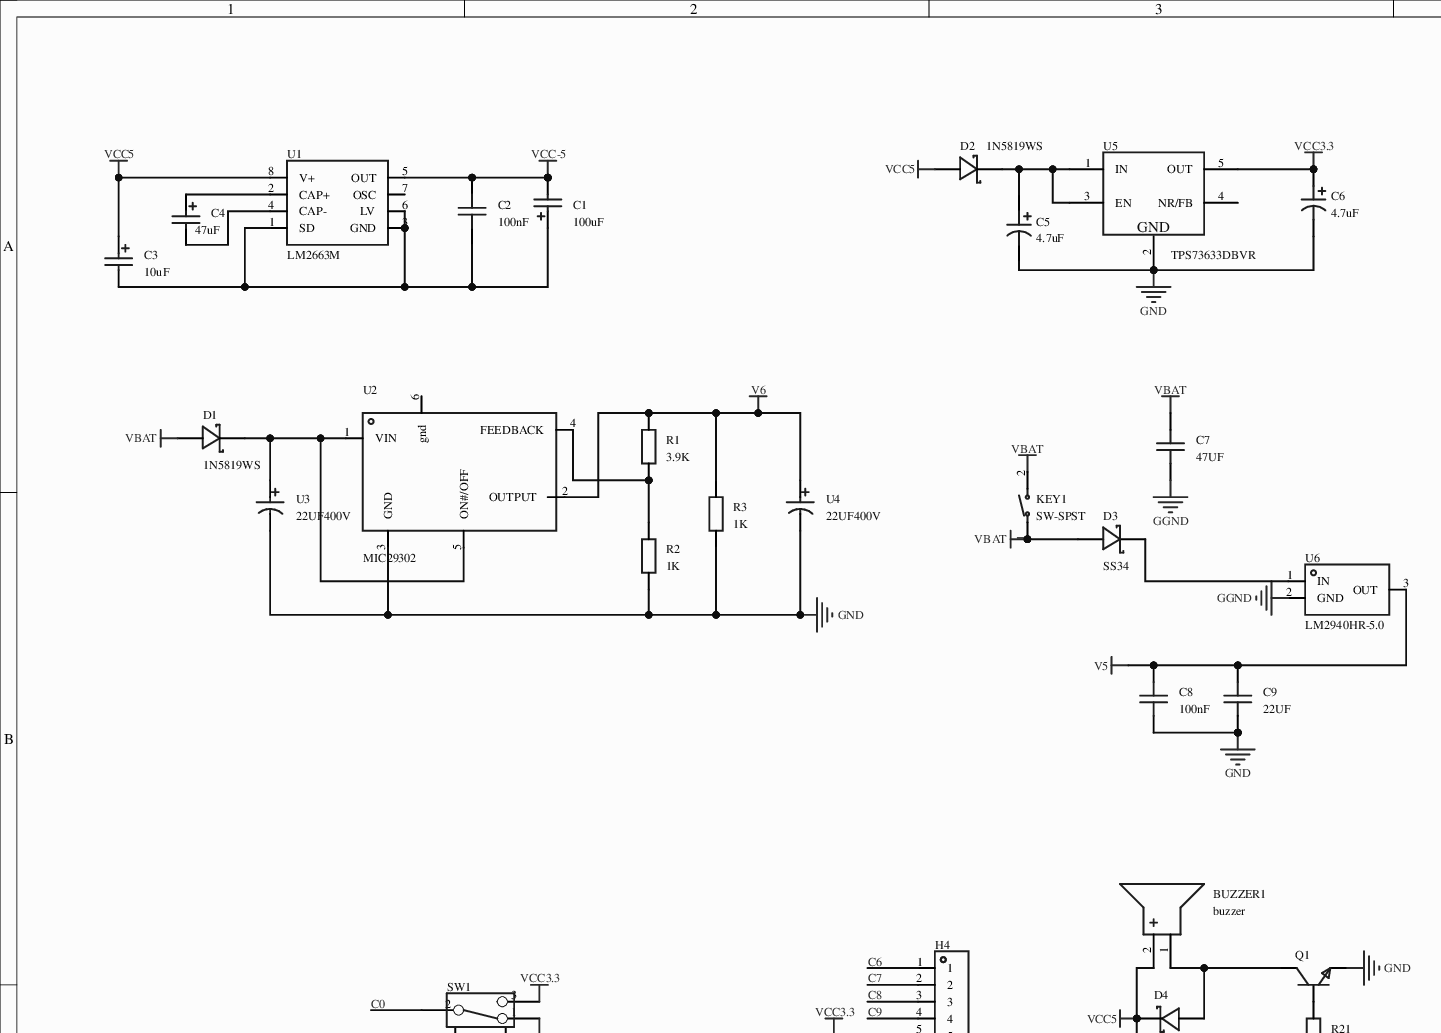
[diagram p0: MISC75407-3.schdoc, top left]
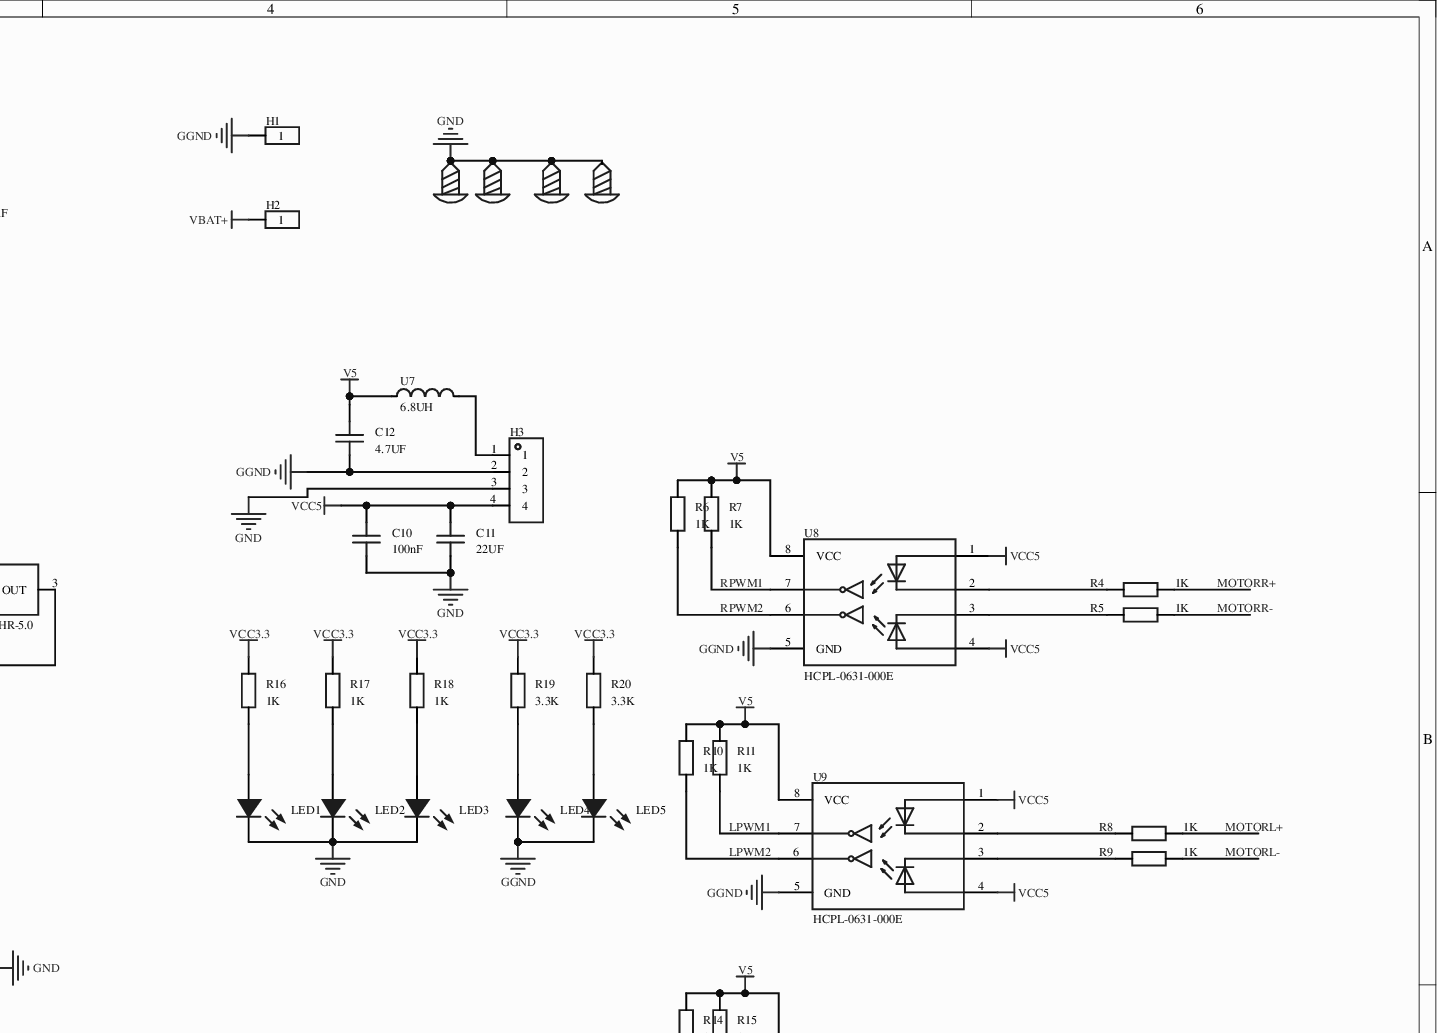
[diagram p1: MISC75407-3.schdoc, top right]
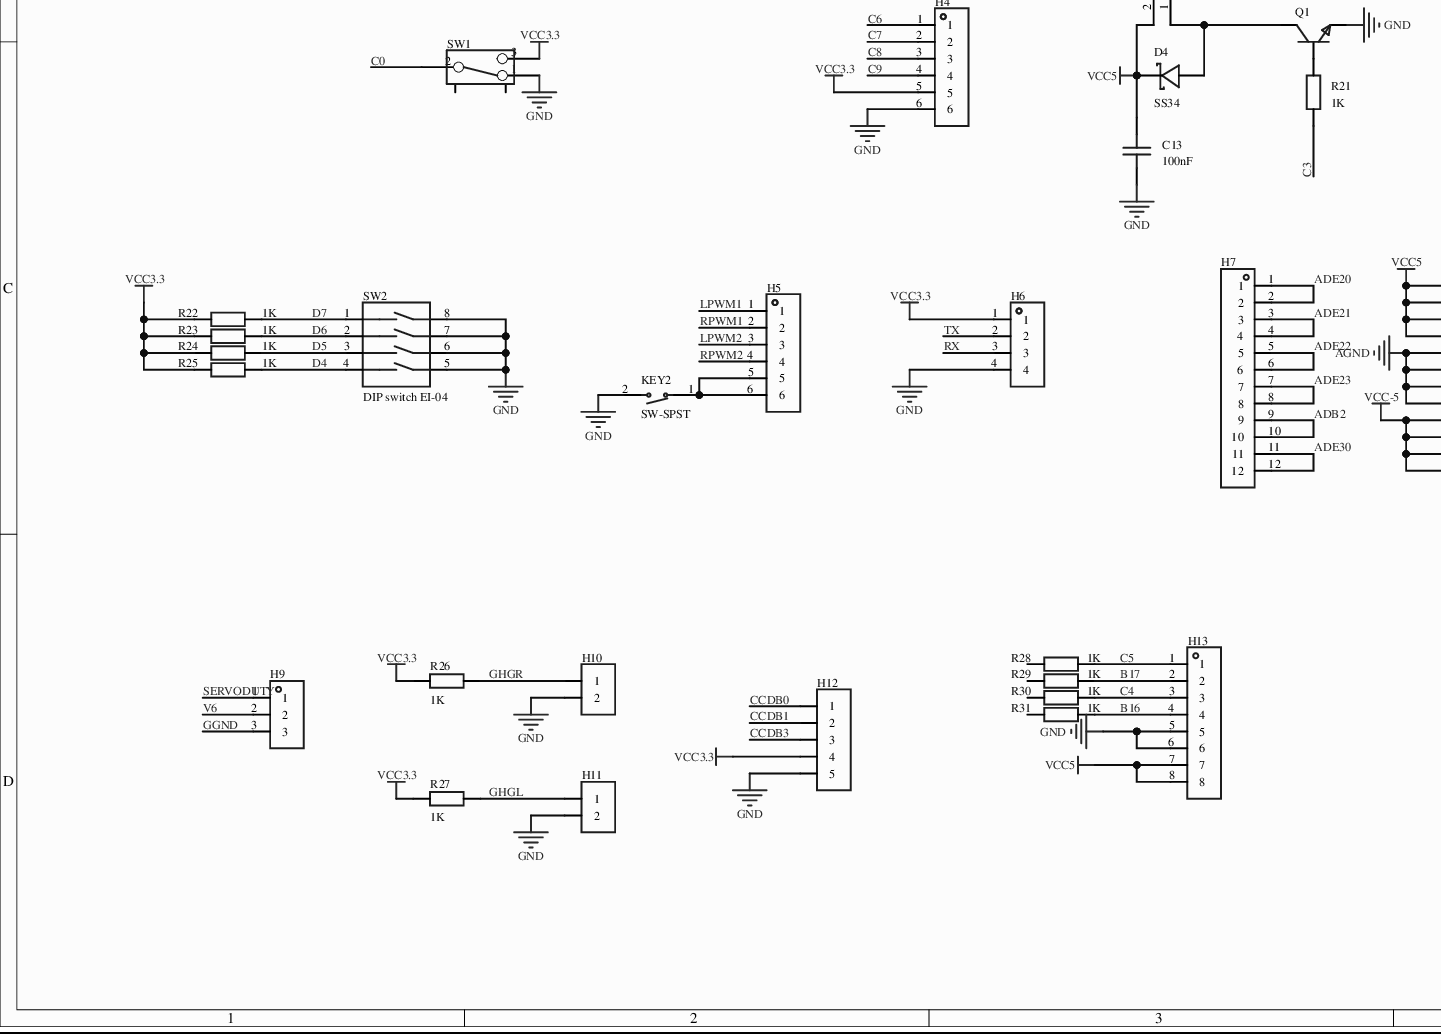
[diagram p2: MISC75407-3.schdoc, bottom left]
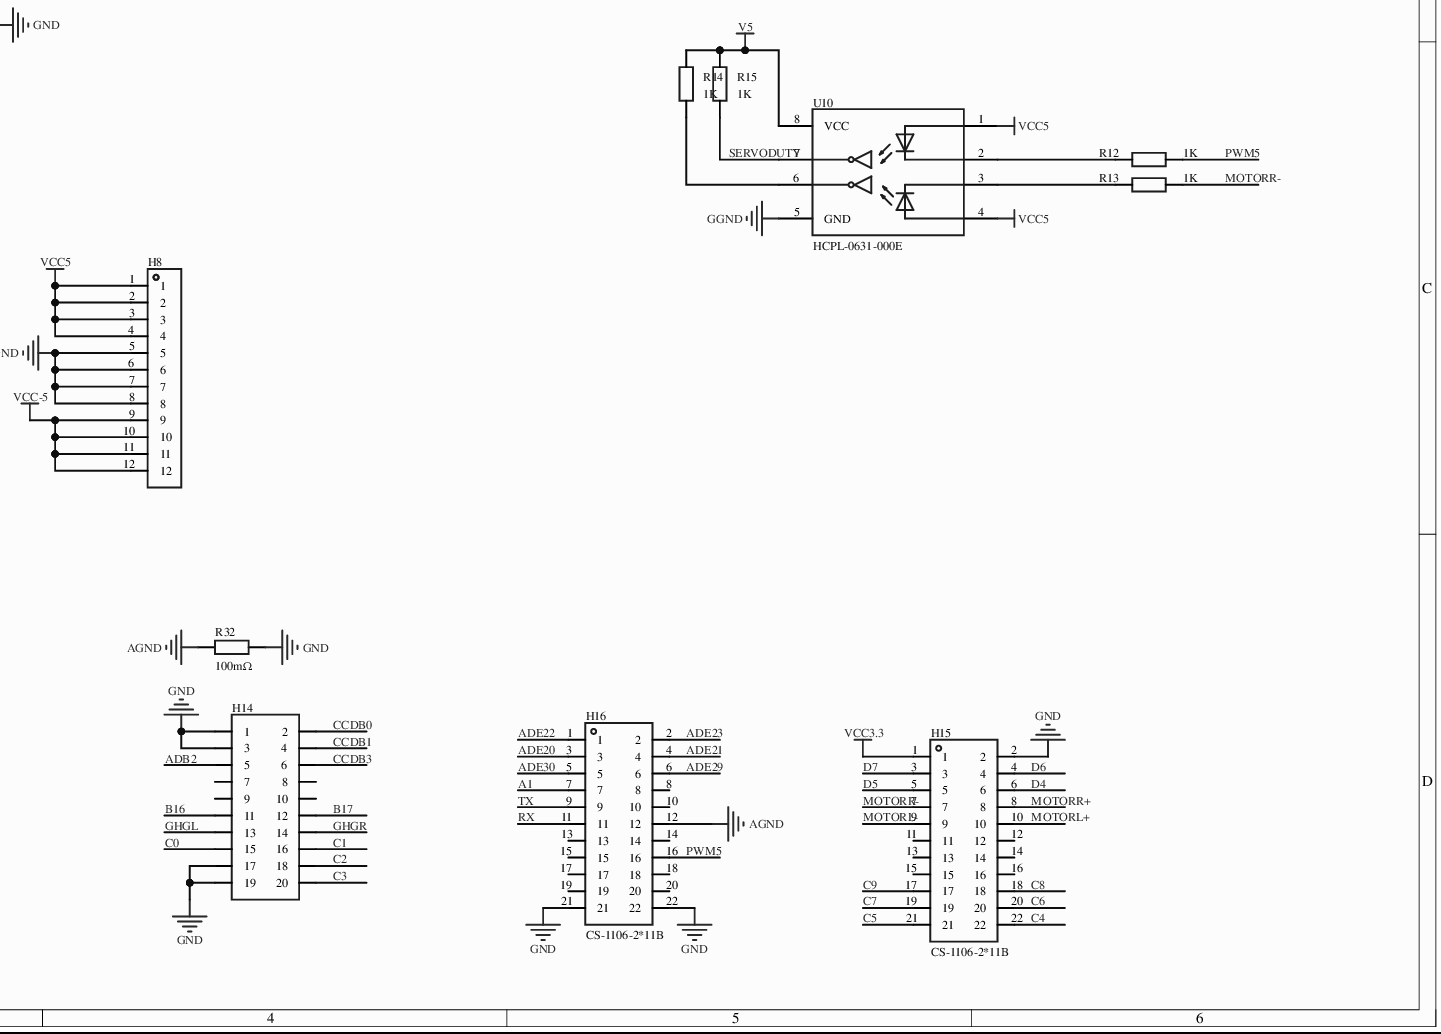
[diagram p3: MISC75407-3.schdoc, bottom right]
# Altium project MISC75407-2.PrjPcb
1 sheet, 90 parts. Net scope: global (net labels, ports and power ports of the same name join across sheets).
Board file: MISC75407.pcbdoc

## Sheet MISC75407-3.schdoc
size 420 x 297 mm; Version: V1.0; @Project Name: MISC75407; @Update Date: 2026-03-22; @Create Date: 2026-03-22; @Board Name: MISC75407; @Create Time: 21:34:52; @Page Count: 1; @Page No: 1; @Schematic Name: MISC75407; @Update Time: 21:34:52; Size: A4

### Parts
BUZZER1  buzzer  [BUZ-TH_BD12.0-P6.00-D0.9-RD]
C1  100uF  [C_Ele_SMD_3x5.4mm]
C2  100nF  [C0603]
C3  10uF  [C_Ele_SMD_3x5.4mm]
C4  47uF  [C_Ele_SMD_3x5.4mm]
C5  4.7uF  [CAP-TH_BD8.0-P3.50-D0.5-FD_4.7UF400V8X14FS]
C6  4.7uF  [CAP-TH_BD8.0-P3.50-D0.5-FD_4.7UF400V8X14FS]
C7  47UF  [C1206]
C8  100nF  [C0603]
C9  22UF  [C1206]
C10  100nF  [C0603]
C11  22UF  [C1206]
C12  4.7UF  [C0603]
C13  100nF  [C0603]
D1  1N5819WS  [SOD-323_L1.8-W1.3-LS2.5-RD]
D2  1N5819WS  [SOD-323_L1.8-W1.3-LS2.5-RD]
D3  SS34  [SMA_L4.3-W2.6-LS5.2-RD]
D4  SS34  [SMA_L4.3-W2.6-LS5.0-RD]
H1  (no value)  [HDR-TH_1P-V-M_XKB_X4611WV-01I-C28D40]
H2  (no value)  [HDR-TH_1P-V-M_XKB_X4611WV-01I-C28D40]
H3  (no value)  [HDR-TH_4P-P2.54-V-F]
H4  (no value)  [HDR-TH_6P-P2.54-V-F]
H5  (no value)  [HDR-TH_6P-P2.54-V-F]
H6  (no value)  [HDR-TH_4P-P2.54-V-F]
H7  (no value)  [HDR-TH_12P-P2.54-V-F]
H8  (no value)  [HDR-TH_12P-P2.54-V-F]
H9  (no value)  [HDR-TH_3P-P2.54-V-F]
H10  (no value)  [HDR-TH_2P-P2.54-V-F]
H11  (no value)  [HDR-TH_2P-P2.54-V-F]
H12  (no value)  [HDR-TH_5P-P2.54-V-F]
H13  (no value)  [HDR-TH_8P-P2.54-V-F-1]
H14  (no value)  [HDR-TH_20P-P2.54-V-R2-C10-S2.54]
H15  CS-1106-2*11B  [HDR-TH_22P-P2.54-V-M-R2-C11-S2.54-1]
H16  CS-1106-2*11B  [HDR-TH_22P-P2.54-V-M-R2-C11-S2.54-1]
KEY1  SW-SPST  [KEY-SMD_L6.0-W3.6-LS8.0]
KEY2  SW-SPST  [KEY-SMD_L6.0-W3.6-LS8.0]
LED1  (no value)  [LED-TH_5mm]
LED2  (no value)  [LED-TH_5mm]
LED3  (no value)  [LED-TH_5mm]
LED4  (no value)  [LED-TH_5mm]
LED5  (no value)  [LED-TH_5mm]
Q1  (no value)  [S8050_TO_92]
R1  3.9K  [R0603]
R2  1K  [R0603]
R3  1K  [R0603]
R4  1K  [R0603]
R5  1K  [R0603]
R6  1K  [R0603]
R7  1K  [R0603]
R8  1K  [R0603]
R9  1K  [R0603]
R10  1K  [R0603]
R11  1K  [R0603]
R12  1K  [R0603]
R13  1K  [R0603]
R14  1K  [R0603]
R15  1K  [R0603]
R16  1K  [R0603]
R17  1K  [R0603]
R18  1K  [R0603]
R19  3.3K  [R0603]
R20  3.3K  [R0603]
R21  1K  [R0603]
R22  1K  [R0603]
R23  1K  [R0603]
R24  1K  [R0603]
R25  1K  [R0603]
R26  1K  [R0603]
R27  1K  [R0603]
R28  1K  [R0603]
R29  1K  [R0603]
R30  1K  [R0603]
R31  1K  [R0603]
R32  100mΩ  [R1206]
SCREW1  (no value)  [M2螺丝]
SCREW2  (no value)  [M2螺丝]
SCREW3  (no value)  [M2螺丝]
SCREW4  (no value)  [M2螺丝]
SW1  (no value)  [拨动开关]
SW2  DIP switch EI-04  [SW-TH_DIPSWITCHEI-04]
U1  LM2663M  [SOIC-8_L4.9-W3.9-P1.27-LS6.0-BL]
U2  MIC29302  [TO-263-5_L10.1-W8.7-P1.70-LS15.2-BR]
U3  22UF400V  [CAP-TH_BD8.0-P3.50-D0.6-FD]
U4  22UF400V  [CAP-TH_BD8.0-P3.50-D0.6-FD]
U5  TPS73633DBVR  [SOT-23-5_L3.0-W1.7-P0.95-LS2.8-BR]
U6  LM2940HR-5.0  [TO-263-2_L10.1-W9.1-P5.08-LS15.2-BR]
U7  6.8UH  [IND-SMD_L10.9-W10.0_ACL1009]
U8  HCPL-0631-000E  [SO-8_L5.1-W3.9-P1.27-LS6.0-BL]
U9  HCPL-0631-000E  [SO-8_L5.1-W3.9-P1.27-LS6.0-BL]
U10  HCPL-0631-000E  [SO-8_L5.1-W3.9-P1.27-LS6.0-BL]

### Nets
AGND: H8.5 H8.6 H8.7 H8.8 H16.12 R32.1
GGND: C7.2 C12.1 H1.1 H3.2 H9.3 LED4.2(A) LED5.2(A) U6.2(GND) U8.5(GND) U9.5(GND) U10.5(GND)
GND: C5.2 C6.2 C8.1 C9.1 C10.1 C11.1 C13.1 H3.3 H4.6 H6.4 H10.2 H11.2 H12.5 H13.5 H13.6 H14.1 H14.3 H14.17 H14.19 H15.2 H16.21 H16.22 KEY2.2 LED1.2(A) LED2.2(A) LED3.2(A) Q1.1(E) R2.1 R3.1 R32.2 SCREW1.1 SCREW2.1 SCREW3.1 SCREW4.1 SW1.1 SW2.5 SW2.6 SW2.7 SW2.8 U2.3(GND) U3.2 U4.2 U5.2(GND)
V5: C8.2 C9.2 C12.2 R6.2 R7.2 R10.2 R11.2 R14.2 R15.2 U6.3(OUT) U7.1 U8.8(VCC) U9.8(VCC) U10.8(VCC)
V6: H9.2 R1.2 R3.2 U2.2(OUTPUT) U4.1
VBAT: C7.1 D1.2(A) D3.2(A) KEY1.1 KEY1.2
VBAT+: H2.1
VCC3.3: C6.1 H4.5 H6.1 H12.4 H15.1 R16.2 R17.2 R18.2 R19.2 R20.2 R22.1 R23.1 R24.1 R25.1 R26.1 R27.1 SW1.3 U5.5(OUT)
VCC5: BUZZER1.2(+) C3.1 C10.2 C11.2 C13.2 D2.2(A) D4.1(K) H3.4 H8.1 H8.2 H8.3 H8.4 H13.7 H13.8 U1.8(V+) U8.1(AN1) U8.4(AN2) U9.1(AN1) U9.4(AN2) U10.1(AN1) U10.4(AN2)
VCC-5: C1.2 C2.2 H8.9 H8.10 H8.11 H8.12 U1.5(OUT)
A1: H16.7
ADB2: H7.9 H7.10 H14.5
ADE20: H7.1 H7.2 H16.3
ADE21: H7.3 H7.4 H16.4
ADE22: H7.5 H7.6 H16.1
ADE23: H7.7 H7.8 H16.2
ADE29: H16.6
ADE30: H7.11 H7.12 H16.5
B16: H13.4 H14.11 R31.2
B17: H13.2 H14.12 R29.2
C0: H14.15 SW1.2
C1: H14.16
C2: H14.18
C3: H14.20 R21.1
C4: H13.3 H15.22 R30.2
C5: H13.1 H15.21 R28.2
C6: H4.1 H15.20
C7: H4.2 H15.19
C8: H4.3 H15.18
C9: H4.4 H15.17
CCDB0: H12.1 H14.2
CCDB1: H12.2 H14.4
CCDB3: H12.3 H14.6
D4: H15.6 R25.2 SW2.4
D5: H15.5 R24.2 SW2.3
D6: H15.4 R23.2 SW2.2
D7: H15.3 R22.2 SW2.1
GHGL: H11.1 H14.13 R27.2
GHGR: H10.1 H14.14 R26.2
LPWM1: H5.1 R11.1 U9.7(VO1)
LPWM2: H5.3 R10.1 U9.6(VO2)
MOTORL+: H15.10 R8.2
MOTORL-: H15.9 R9.2
MOTORR+: H15.8 R4.2
MOTORR-: H15.7 R5.2 R13.2
PWM5: H16.16 R12.2
RPWM1: H5.2 R7.1 U8.7(VO1)
RPWM2: H5.4 R6.1 U8.6(VO2)
RX: H6.3 H16.11
SERVODUTY: H9.1 R15.1 U10.7(VO1)
TX: H6.2 H16.9
NetBUZZER1_1: BUZZER1.1(-) D4.2(A) Q1.3(C)
NetC1_1: C1.1 C2.1 C3.2 U1.1(SD) U1.3(GND) U1.6(LV)
NetC4_1: C4.1 U1.2(CAP+)
NetC4_2: C4.2 U1.4(CAP-)
NetC5_1: C5.1 D2.1(K) U5.1(IN) U5.3(EN)
NetD1_1: D1.1(K) U2.1(VIN) U2.5(ON#/OFF) U3.1
NetD3_1: D3.1(K) U6.1(IN)
NetH3_1: H3.1 U7.2
NetH5_5: H5.5 H5.6 KEY2.1
NetLED1_1: LED1.1(C) R16.1
NetLED2_1: LED2.1(C) R17.1
NetLED3_1: LED3.1(C) R18.1
NetLED4_1: LED4.1(C) R19.1
NetLED5_1: LED5.1(C) R20.1
NetQ1_2: Q1.2(B) R21.2
NetR1_1: R1.1 R2.2 U2.4(FEEDBACK)
NetR4_1: R4.1 U8.2(CAT1)
NetR5_1: R5.1 U8.3(CAT2)
NetR8_1: R8.1 U9.2(CAT1)
NetR9_1: R9.1 U9.3(CAT2)
NetR12_1: R12.1 U10.2(CAT1)
NetR13_1: R13.1 U10.3(CAT2)
NetR14_1: R14.1 U10.6(VO2)

Not connected (* = marked no-connect by the designer): H14 7* 8* 9* 10*; H15 11* 12* 13* 14* 15* 16*; H16 8* 10* 13* 14* 15* 17* 18* 19* 20*; R28 1; R29 1; R30 1; R31 1; SW1 4 5; U1 7(OSC); U2 6(gnd); U5 4(NR/FB)

### Library data of the parts
BUZZER1 = buzzer: AddInBom: yes; ModelId: af17e4151ed84fc2a628230bf23763630819f05c4eef4c71ace90d822a990e87; ModelTransform: 472.44,472.176,0,270,0,0,0,0,-196.85; Symbol: BUZZER; Device: buzzer; LCSC Part Name: buzzer; SupplierPart: C9900014030; ManufacturerPart: buzzer; Supplier Footprint: buzzer; JLCPCB Part Class: Extended Part; Supplier: LCSC; ConvertToPcb: yes; FootprintName: BUZ-TH_BD12.0-P6.00-D0.9-RD; ModelName: BUZ-TH_BD12.0-P6.00-D0.9-RD
C1 C3 C4 = C_Ele_SMD_3x5.4mm: Symbol: CAP; AddInBom: yes; ModelId: 0132c3d3fdbf4fd987f710a97e7a5b5d0819f05c4eef4c71ace90d822a990e87; ModelName: CAP-SMD_BD3.0-L3.3-W3.3-H5.3; ModelTransform: 129.9,149.58,209.06,-90,0,0,0,0,0; Device: C_Ele_SMD_3x5.4mm; Supplier Footprint: SMD,3x5.4mm; ConvertToPcb: yes; FootprintName: C_Ele_SMD_3x5.4mm
  C1: Value: 100uF
  C3: Value: 10uF
  C4: Value: 47uF
C2 C8 C10 C12 C13 = CAP_0603: Symbol: Capacitance; ConvertToPcb: yes; ModelId: ac125912035d415993ca9572d50418b10819f05c4eef4c71ace90d822a990e87; ModelName: C0603_L1.6-W0.8-H0.8; ModelTransform: 62.992,31.496,0,0,0,0,0,0,0; Device: CAP_0603; AddInBom: yes; Supplier Footprint: 0603; FootprintName: C0603
  C2 C8 C10 C13: Value: 100nF
  C12: Value: 4.7UF
C5 C6 = 4.7uF400V8x14FS: Capacitance: 4.7uF; tolerance: ±20%; rated voltage: 400V; ripple current: 220mA@100KHz; equivalent series resistance (ESR): 11Ω;; Manufacturer: Econd(米朗电子); AddInBom: yes; Pin Spacing: 2.5mm; Lifetime: 5000hrs@105℃; Symbol: 4.7UF400V8X14FS; Device: 4.7uF400V8x14FS; LCSC Part Name: 4.7uF ±20% 400V; SupplierPart: C49304883; ManufacturerPart: 4.7uF400V8x14FS; Supplier Footprint: 插件,D8xL14mm; JLCPCB Part Class: Extended Part; Datasheet: https://item.szlcsc.com/datasheet/4.7uF400V8x14FS/51766711.html; Supplier: LCSC; ConvertToPcb: yes; FootprintName: CAP-TH_BD8.0-P3.50-D0.5-FD_4.7UF400V8X14FS; Value: 4.7uF; Tolerance: ±20%; Voltage Rating: 400V; Ripple Current: 220mA@100KHz; Equivalent Series Resistance(ESR): 11Ω; Diameter: 8mm; Height - Seated (Max): 14mm; Operating Temperature: -25℃~+105℃
C7 = 47UF: AddInBom: yes; ModelId: e4be705b945545a48e666415e3682bd80819f05c4eef4c71ace90d822a990e87; ModelName: C1206_L3.2-W1.6-H1.3; ModelTransform: 125.984,62.992,0,0,0,0,0,0,0; Symbol: 47UF; Device: 47UF; LCSC Part Name: 47UF; SupplierPart: C9900009812; ManufacturerPart: 47UF; Supplier Footprint: C1206; JLCPCB Part Class: Extended Part; Supplier: LCSC; ConvertToPcb: yes; FootprintName: C1206
C9 C11 = 22UF: Symbol: 22UF_C9900008064; AddInBom: yes; ModelId: e4be705b945545a48e666415e3682bd80819f05c4eef4c71ace90d822a990e87; ModelName: C1206_L3.2-W1.6-H1.3; ModelTransform: 125.984,62.992,0,0,0,0,0,0,0; Device: 22UF; LCSC Part Name: 22UF; SupplierPart: C9900008064; ManufacturerPart: 22UF; Supplier Footprint: 1206; JLCPCB Part Class: Extended Part; Supplier: LCSC; ConvertToPcb: yes; FootprintName: C1206
D1 D2 = 1N5819WS_C191023: Forward voltage (Vf): 600mV@1A; DC reverse voltage (Vr): 40V; rectified current: 1A;; Manufacturer: Hottech(合科泰); AddInBom: yes; ModelId: 7459fe65e23146c0a8d836e46a0add720819f05c4eef4c71ace90d822a990e87; ModelTransform: 104.3305,51.181,0,0,0,0,0,0,0; Non-Repetitive Peak Forward Surge Current: 25A; Symbol: 1N5819WS; Device: 1N5819WS_C191023; LCSC Part Name: 电压:40V 电流:1A; SupplierPart: C191023; ManufacturerPart: 1N5819WS; Supplier Footprint: SOD-323; JLCPCB Part Class: Basic Part; Datasheet: https://item.szlcsc.com/datasheet/1N5819WS/213850.html; Supplier: LCSC; ConvertToPcb: yes; FootprintName: SOD-323_L1.8-W1.3-LS2.5-RD; ModelName: SOD-323_L1.8-W1.3-LS2.5-RD; Voltage - Forward(Vf@If): 600mV@1A; Voltage - DC Reverse(Vr): 40V; Current - Rectified: 1A
D3 = SS34_C8678: Diode configuration: single; forward voltage (Vf): 550mV@3A; DC reverse voltage (Vr): 40V; rectified current: 3A;; Manufacturer: MDD(辰达半导体); AddInBom: yes; ModelId: e3551acb3c5a4975a5e9d36087fe1fa20819f05c4eef4c71ace90d822a990e87; ModelTransform: 185.039,102.362,0,0,0,0,0,0,0; Reverse Leakage Current (Ir): 500uA@40V; Operating Junction Temperature Range: -55℃~+125℃; Symbol: SS34_C8678; Device: SS34_C8678; LCSC Part Name: 电压:40V 电流:3A; SupplierPart: C8678; ManufacturerPart: SS34; Supplier Footprint: SMA(DO-214AC); JLCPCB Part Class: Basic Part; Datasheet: https://item.szlcsc.com/datasheet/SS34/9178.html; Supplier: LCSC; ConvertToPcb: yes; FootprintName: SMA_L4.3-W2.6-LS5.2-RD; ModelName: SMA_L4.3-W2.6-LS5.2-RD; Diode Configuration: Single; Voltage - Forward(Vf@If): 550mV@3A; Voltage - DC Reverse(Vr): 40V; Current - Rectified: 3A
D4 = SS34: Symbol: SS34_C9900023345; AddInBom: yes; ModelId: 8d2dd2e50a3a4b27821fa63d469a8f110819f05c4eef4c71ace90d822a990e87; ModelTransform: 196.85,102.362,0,0,0,0,0,0,0; Device: SS34; LCSC Part Name: SS34; SupplierPart: C9900023345; ManufacturerPart: SS34; Supplier Footprint: SMA,DO-214AC; JLCPCB Part Class: Extended Part; Supplier: LCSC; ConvertToPcb: yes; FootprintName: SMA_L4.3-W2.6-LS5.0-RD; ModelName: SMA_L4.3-W2.6-LS5.0-RD
H1 H2 = HDR-M_2.54_1x1P: Symbol: HDR_1x1; ConvertToPcb: yes; ModelId: 95857080d3cc4057a19a22ccce05e1710819f05c4eef4c71ace90d822a990e87; ModelTransform: 78.74,79.1337,0,0,0,0,0,0,-110.236; Device: HDR-M_2.54_1x1P; AddInBom: yes; SupplierPart: C81276; Supplier Footprint: 插件; FootprintName: HDR-TH_1P-V-M_XKB_X4611WV-01I-C28D40; JLCPCB Part Class: Extended Part; ModelName: HDR-TH_1P-V-M_XKB_X4611WV-01I-C28D40
H3 H6 = HDR-F_2.54_1x4P: Symbol: 2.54-1*4P female; ConvertToPcb: yes; ModelId: d187812051054f85879fcaa51a310d8e0819f05c4eef4c71ace90d822a990e87; ModelTransform: 419.6842,98.464,0,0,0,0,0,0,-118.11; Device: HDR-F_2.54_1x4P; AddInBom: yes; SupplierPart: C2718488; Supplier Footprint: 插件; FootprintName: HDR-TH_4P-P2.54-V-F; ModelName: HDR-TH_4P-P2.54-V-F
H4 H5 = HDR-F_2.54_1x6P: Symbol: Header-Female-2.54_1x6; ConvertToPcb: yes; ModelId: 0f5bcf94dcda47d085f24cdca1696fe90819f05c4eef4c71ace90d822a990e87; ModelTransform: 619.684,94.488,0,0,0,0,0,0,-125.984; Device: HDR-F_2.54_1x6P; AddInBom: yes; SupplierPart: C40877; Supplier Footprint: 插件; FootprintName: HDR-TH_6P-P2.54-V-F; ModelName: HDR-TH_6P-P2.54-V-F
H7 H8 = HDR-F_2.54_1x12P: ConvertToPcb: yes; ModelId: a8b4b2347edc4eeab5667ae97bf18e170819f05c4eef4c71ace90d822a990e87; ModelName: HDR-TH_12P-P2.54-F-LI-1X12P; ModelTransform: 1215.74568,98.425,0,0,0,0,0,0,-129.921; Symbol: HDR-F_2.54_1x12P; Device: HDR-F_2.54_1x12P; AddInBom: yes; SupplierPart: C2905419; Supplier Footprint: 插件; FootprintName: HDR-TH_12P-P2.54-V-F
H9 = HDR-F_2.54_1x3P: Symbol: PM254V-11-03-H85; ConvertToPcb: yes; ModelId: f3b3cc5aae9641bf9e56fc160cef875b0819f05c4eef4c71ace90d822a990e87; ModelName: HDR2.54-F-LI-1X3P; ModelTransform: 299.9994,100,0,0,0,0,0,0,-118.11; Device: HDR-F_2.54_1x3P; AddInBom: yes; SupplierPart: C541850; Supplier Footprint: 插件; FootprintName: HDR-TH_3P-P2.54-V-F
H10 H11 = HDR-F_2.54_1x2P: Symbol: Header-Female-2.54_1x2; ConvertToPcb: yes; ModelId: a9450ef445564560a104363b9aacde4e0819f05c4eef4c71ace90d822a990e87; ModelName: HDR-TH_2P-P2.54-F-LI-1X2P; ModelTransform: 215.7476,98.425,0,0,0,0,0,0,-129.921; Device: HDR-F_2.54_1x2P; AddInBom: yes; SupplierPart: C49661; Supplier Footprint: 插件; FootprintName: HDR-TH_2P-P2.54-V-F
H12 = HDR-F_2.54_1x5P: Symbol: Header-Female-2.54_1x5; ConvertToPcb: yes; ModelId: f49cb6116a3d45e5a64915bf3e00773f0819f05c4eef4c71ace90d822a990e87; ModelTransform: 519.684,98.464,0,0,0,0,0,0,-124.016; Device: HDR-F_2.54_1x5P; AddInBom: yes; SupplierPart: C50950; Supplier Footprint: 插件; FootprintName: HDR-TH_5P-P2.54-V-F; ModelName: HDR-TH_5P-P2.54-V-F
H13 = HDR-F_2.54_1x8P: Symbol: Header-Female-2.54_1x8; AddInBom: yes; ModelId: 0f7e4d9227ef4fa08d5469c22cc70cdb0819f05c4eef4c71ace90d822a990e87; ModelName: HDR-F-2.54_1x8; ModelTransform: 799.99844,100,0,0,0,0,0,0,-118.11; Device: HDR-F_2.54_1x8P; ConvertToPcb: yes; FootprintName: HDR-TH_8P-P2.54-V-F-1; SupplierPart: C27438; Supplier Footprint: 插件
H14 = HDR-F_2.54_2x10: Symbol: HDR-F-2.54_2x10; ConvertToPcb: yes; ModelId: e61a236d230547b1b0067fd6f2acc5ad0819f05c4eef4c71ace90d822a990e87; ModelTransform: 999.99796,200,0,0,0,0,0,0,-118.11; Device: HDR-F_2.54_2x10; AddInBom: yes; SupplierPart: C30867; Supplier Footprint: 插件; FootprintName: HDR-TH_20P-P2.54-V-R2-C10-S2.54; ModelName: HDR-F-2.54_2x10
H15 H16 = CS-1106-2*11B: Pin structure: 2x11P; pitch: 2.54mm; row spacing: 2.54mm; round/square pin: square pin; mounting: through-hole; rows: dual row; total pin count: 22P; rated current: 3A; rated voltage: 250V; mating pin length: 6.9mm; plastic height: -; tail length: 3mm; contact material: -; operating temperature: -40℃~+105℃; colour: -;; Manufacturer: CST(永丰盈); AddInBom: yes; ModelId: 07268b35c943498bbe3db8a4859c2fb20819f05c4eef4c71ace90d822a990e87; ModelTransform: 1100.39146,196.85,0,0,0,0,0,0,-98.425; Symbol: CS-1106-2*11B; Device: CS-1106-2*11B; LCSC Part Name: 2x11P 间距:2.54mm 方针 直插; SupplierPart: C2886715; ManufacturerPart: CS-1106-2*11B; Supplier Footprint: 插件,P=2.54mm; JLCPCB Part Class: Extended Part; Datasheet: https://atta.szlcsc.com/upload/public/pdf/source/20210907/581D023C58564783982DEC168A9328C8.pdf; Supplier: LCSC; ConvertToPcb: yes; FootprintName: HDR-TH_22P-P2.54-V-M-R2-C11-S2.54-1; ModelName: HDR-TH_22P-P2.54-V-M-R2-C11-S2.54-1; Pin Structure: 2x11P; Pitch: 2.54mm; Row Spacing: 2.54mm; Circluar Pins/Square Pins: Square pin; Mounting Type: Through-hole; Number of Rows: Dual row; Number of Pins: 22P; Current Rating: 3A; Voltage Rating (Max): 250V; Length of Mating Pin: 6.9mm; Insulation Height: -; Length of End Connection Pin: 3mm; Contact Material: -; Operating Temperature: -40℃~+105℃; Color: -
KEY1 KEY2 = SW-SPST-SMT3*6*2.5贴片按钮: Symbol: SW-SPST-SMT3*6*2.5 SMD push button; AddInBom: yes; ModelId: 0f725c733cf24d50be61650f948fb9ee0819f05c4eef4c71ace90d822a990e87; ModelTransform: 314.96,141.732,0,0,0,0,0.004,-0.002,0; Device: SW-SPST-SMT3*6*2.5 SMD push button; Manufacturer Part: SW-SPST; LCSC Part Name: SW-SPST-SMT3*6*2.5贴片按钮; SupplierPart: C9900003180; Supplier Footprint: SMD_L6.0-W3.6-LS8.0; JLCPCB Part Class: Extended Part; Supplier: LCSC; ConvertToPcb: yes; FootprintName: KEY-SMD_L6.0-W3.6-LS8.0; ModelName: KEY-SMD_L6.0-W3.6-LS8.0
LED1-LED5 = LED_TH-B_5mm: AddInBom: yes; ModelId: b0e300213b7e4bc9906214592eb37e0a0819f05c4eef4c71ace90d822a990e87; ModelName: LED-TH_BD5.0_Blue; ModelTransform: 177.89258,177.84487,480.30997,90,0,0,-1.9685,0,-389.76378; Symbol: LED_TH-B; Device: LED_TH-B_5mm; ConvertToPcb: yes; FootprintName: LED-TH_5mm; Supplier Footprint: 插件
Q1 = S8050_TO_NPN: ConvertToPcb: yes; ModelId: aafe8e06f2154e7c93506efd0d6632dd0819f05c4eef4c71ace90d822a990e87; ModelName: TO-92-3_L4.9-W3.7-P1.27-L; ModelTransform: 180.78,141.44,417.3,0,0,0,0,0,-200; Symbol: S8050_TO_NPN; Device: S8050_TO_NPN; AddInBom: yes; Supplier Footprint: TO-92; FootprintName: S8050_TO_92
R1-R31 = Res_0603: Symbol: Resistor; ConvertToPcb: yes; ModelId: fc143cca1e79419f9cd78b61e9279f080819f05c4eef4c71ace90d822a990e87; ModelTransform: 31.8897,63.7794,0,90,0,0,0,0,0; Device: Res_0603; AddInBom: yes; Supplier Footprint: 0603; FootprintName: R0603; ModelName: R0603
  R1: Value: 3.9K
  R2-R18 R21-R31: Value: 1K
  R19 R20: Value: 3.3K
R32 = 1206W4F100LT5E: Resistor type: thick film resistor; resistance: 100mΩ; tolerance: ±1%; power: 250mW; operating voltage: 200V; temperature coefficient: ±800ppm/℃;; Manufacturer: UNI-ROYAL(厚声); AddInBom: yes; ModelId: 89a1f13db2384da588040e0b3c55bf660819f05c4eef4c71ace90d822a990e87; ModelName: R1206_L3.2-W1.6-H0.6; ModelTransform: 125.984,62.992,0,0,0,0,0,0,0; Symbol: 1206W4F100LT5E; Device: 1206W4F100LT5E; LCSC Part Name: 100mΩ ±1% 250mW 厚膜电阻; SupplierPart: C25334; ManufacturerPart: 1206W4F100LT5E; Supplier Footprint: 1206; JLCPCB Part Class: Basic Part; Datasheet: https://item.szlcsc.com/datasheet/1206W4F100LT5E/26077.html; Supplier: LCSC; ConvertToPcb: yes; FootprintName: R1206; Type: Thick film resistor; Value: 100mΩ; Tolerance: ±1%; Power(Watts): 250mW; Voltage-Supply(Max): 200V; Temperature Coefficient: ±800ppm/℃; Operating Temperature: -55℃~+155℃
SCREW1-SCREW4 = M2螺丝: Symbol: Screw hole; Device: M2 screw; ConvertToPcb: yes; AddInBom: yes; Supplier Footprint: 插件; FootprintName: M2 screw
SW1 = 拨动开关_正: Symbol: Toggle switch; Device: Toggle switch_positive; ConvertToPcb: yes; ModelId: 4321fe59a4074cbfb4989553f297c68f0819f05c4eef4c71ace90d822a990e87; ModelName: SW-TH_SS-12D02-VG4; ModelTransform: 370.09,208.7,472.35,0,0,0,0,0,-110; AddInBom: yes; Supplier Footprint: 插件; FootprintName: Toggle switch
SW2 = 拨码开关EI-04: Type: flat lever, raised; circuit structure: SPST; switch positions: 4; service life: -; colour: black;; Manufacturer: 圜达; AddInBom: yes; ModelId: 05004328256048a2b98ea2194ea807530819f05c4eef4c71ace90d822a990e87; ModelName: SW-TH_DIPSWITCHEI-04-L10.1-W6.0-H3.4-P2.54-LS7.6; ModelTransform: 396.0622,309.842,0,0,0,0,0,0,-137.795; Number of Positions: 4 positions; Symbol: DIP switchEI-04; Device: DIP switch EI-04; LCSC Part Name: 拨码开关EI-04; SupplierPart: C99987; ManufacturerPart: 拨码开关EI-04; Supplier Footprint: -; JLCPCB Part Class: Extended Part; Datasheet: https://atta.szlcsc.com/upload/public/pdf/source/20170504/1493892386551.pdf; Supplier: LCSC; ConvertToPcb: yes; FootprintName: SW-TH_DIPSWITCHEI-04; Type: Flat lever, raised; Circuit: SPST; Lead Pitch: 2.54mm; Operating Life: -; Color: Black
U1 = LM2663M: LM2663 200mA switched-capacitor voltage converter with low-current shutdown mode; AddInBom: yes; ModelId: e81d2f7d937b4a6ab1dca543ff5d56a40819f05c4eef4c71ace90d822a990e87; ModelName: SOIC-8_L4.9-W3.9-H1.7-LS6.0-P1.27; ModelTransform: 192.913,236.22,0,0,0,0,0,0,0; Symbol: LM2663M; Device: LM2663M; LCSC Part Name: LM2663M; SupplierPart: C3199749; ManufacturerPart: LM2663M; Supplier Footprint: SOIC-8; JLCPCB Part Class: Extended Part; Datasheet: https://www.ti.com/cn/lit/gpn/lm2663; Supplier: LCSC; ConvertToPcb: yes; FootprintName: SOIC-8_L4.9-W3.9-P1.27-LS6.0-BL
U2 = MIC29302: AddInBom: yes; ModelId: cb803ec6d9174a6189dc62586ef983d20819f05c4eef4c71ace90d822a990e87; ModelTransform: 598.424,397.83385,0,0,0,0,-59.055,0,0; Symbol: MIC29302; Device: MIC29302; LCSC Part Name: MIC29302; SupplierPart: C9900009660; ManufacturerPart: MIC29302; Supplier Footprint: TO-263-5; JLCPCB Part Class: Extended Part; Supplier: LCSC; ConvertToPcb: yes; FootprintName: TO-263-5_L10.1-W8.7-P1.70-LS15.2-BR; ModelName: TO-263-5_L10.1-W8.7-P1.70-LS15.2-BR
U3 U4 = 22UF400V: AddInBom: yes; ModelId: a2c936ec27754f809f3966430e36f7670819f05c4eef4c71ace90d822a990e87; ModelName: CAP-TH_D8.0-H8.0-P3.50; ModelTransform: 314.96,314.862,0,180,0,0,0,0,-137.795; Symbol: 22UF400V; Device: 22UF400V; LCSC Part Name: 22UF400V; SupplierPart: C9900013823; ManufacturerPart: 22UF400V; Supplier Footprint: 22uF400V; JLCPCB Part Class: Extended Part; Supplier: LCSC; ConvertToPcb: yes; FootprintName: CAP-TH_BD8.0-P3.50-D0.6-FD
U5 = TPS73633DBVR: Output type: fixed; max input voltage: 5.5V; output voltage: 3.3V; output current: 400mA; PSRR: 58dB@(100Hz); 37dB@(10kHz); output polarity: positive;; Manufacturer: TI(德州仪器); AddInBom: yes; ModelId: 0a2a1b8f50944f73965918ad6e5fe1670819f05c4eef4c71ace90d822a990e87; ModelName: SOT-23-5_L2.9-W1.6-H1.1-LS2.8-P0.95; ModelTransform: 114.173,109.636,0,180,0,0,0,0,0; Dropout Voltage: 200mV@(400mA); standby current: 550uA; Number of Outputs: 1; Symbol: TPS73633DBVR; Device: TPS73633DBVR; LCSC Part Name: 具有反向电流保护和使能功能的 400mA、高精度、超低压降稳压器; SupplierPart: C28038; ManufacturerPart: TPS73633DBVR; Supplier Footprint: SOT-23-5; JLCPCB Part Class: Extended Part; Datasheet: https://www.ti.com/cn/lit/gpn/tps736; Supplier: LCSC; ConvertToPcb: yes; FootprintName: SOT-23-5_L3.0-W1.7-P0.95-LS2.8-BR; Output Type: Fixed; Maximum Input Voltage: 5.5V; Output Voltage: 3.3V; Output Current: 400mA; Power Supply Rejection Ratio (PSRR): 58dB@(100Hz);37dB@(10kHz); Feature: ESD protection; low ESR; thermal shutdown (TSD); overcurrent protection (OCP); with enable; with charge pump; reverse current protection; Operating Temperature: -40℃~+125℃; Output Polarity: Positive
U6 = LM2940HR-5.0: Manufacturer: HTC; AddInBom: yes; ModelId: d0164c4729fb485ab05f312a49c96c520819f05c4eef4c71ace90d822a990e87; ModelName: TO-263-2_L10.2-W8.7-H4.5-LS15.2-P2.54; ModelTransform: 401.574,591.64307,0,90,0,0,-45.695,0,0; Symbol: LM2940HR-5.0; Device: LM2940HR-5.0; LCSC Part Name: LM2940HR-5.0; SupplierPart: C48705240; ManufacturerPart: LM2940HR-5.0; Supplier Footprint: TO-263-3L; JLCPCB Part Class: Extended Part; Datasheet: https://item.szlcsc.com/datasheet/LM2940HR-5.0/50997115.html; Supplier: LCSC; ConvertToPcb: yes; FootprintName: TO-263-2_L10.1-W9.1-P5.08-LS15.2-BR
U7 = 6.8UH: Symbol: 6.8UH_C9900164995; AddInBom: yes; ModelId: b8b29277a0b64b06905d3086513b7c0a0819f05c4eef4c71ace90d822a990e87; ModelTransform: 429.133,394.094,0,0,0,0,0,0,0; Device: 6.8UH; LCSC Part Name: 6.8UH; SupplierPart: C9900164995; ManufacturerPart: 6.8UH; Supplier Footprint: ACL1009; JLCPCB Part Class: Extended Part; Supplier: LCSC; ConvertToPcb: yes; FootprintName: IND-SMD_L10.9-W10.0_ACL1009; ModelName: IND-SMD_L10.9-W10.0_ACL1009
U8-U10 = HCPL-0631-000E: Input type: DC; operating voltage: 4.5V~5.5V; data rate: 10Mbps;; Manufacturer: Broadcom(博通); AddInBom: yes; ModelId: d496d6c3ca0c4fce912e4076cc25ea7c0819f05c4eef4c71ace90d822a990e87; ModelName: SO-8_L5.1-W4.0-H3.2-P1.27; ModelTransform: 236.454,200.787,0,90,0,0,0,0,0; Isolation Voltage(Vrms): 3.75kV; Number of Channels: 2; Symbol: HCPL-0631-000E; Device: HCPL-0631-000E; LCSC Part Name: DC输入 2通道 隔离电压(rms):3750V; SupplierPart: C188702; ManufacturerPart: HCPL-0631-000E; Supplier Footprint: SO-8; JLCPCB Part Class: Extended Part; Datasheet: https://item.szlcsc.com/datasheet/HCPL-0631-000E/200110.html; Supplier: LCSC; ConvertToPcb: yes; FootprintName: SO-8_L5.1-W3.9-P1.27-LS6.0-BL; Input Type: DC; Voltage - Supply: 4.5V~5.5V; Data Rate: 10Mbps; Operating Temperature: -40℃~+85℃